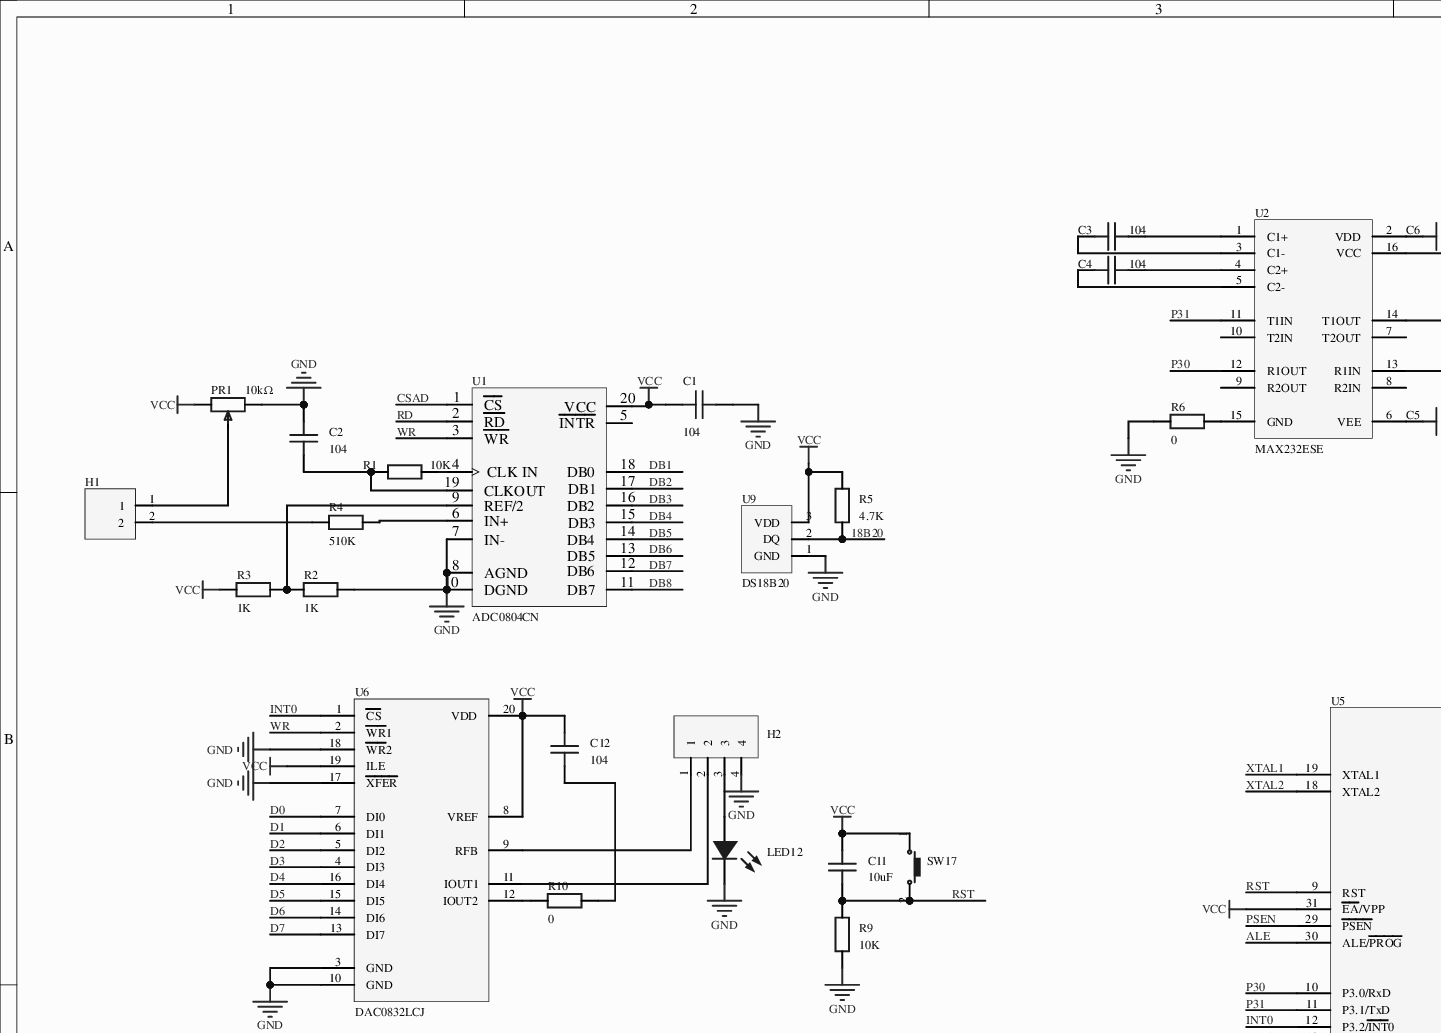
[diagram p0: MISC49866-3.schdoc, top left]
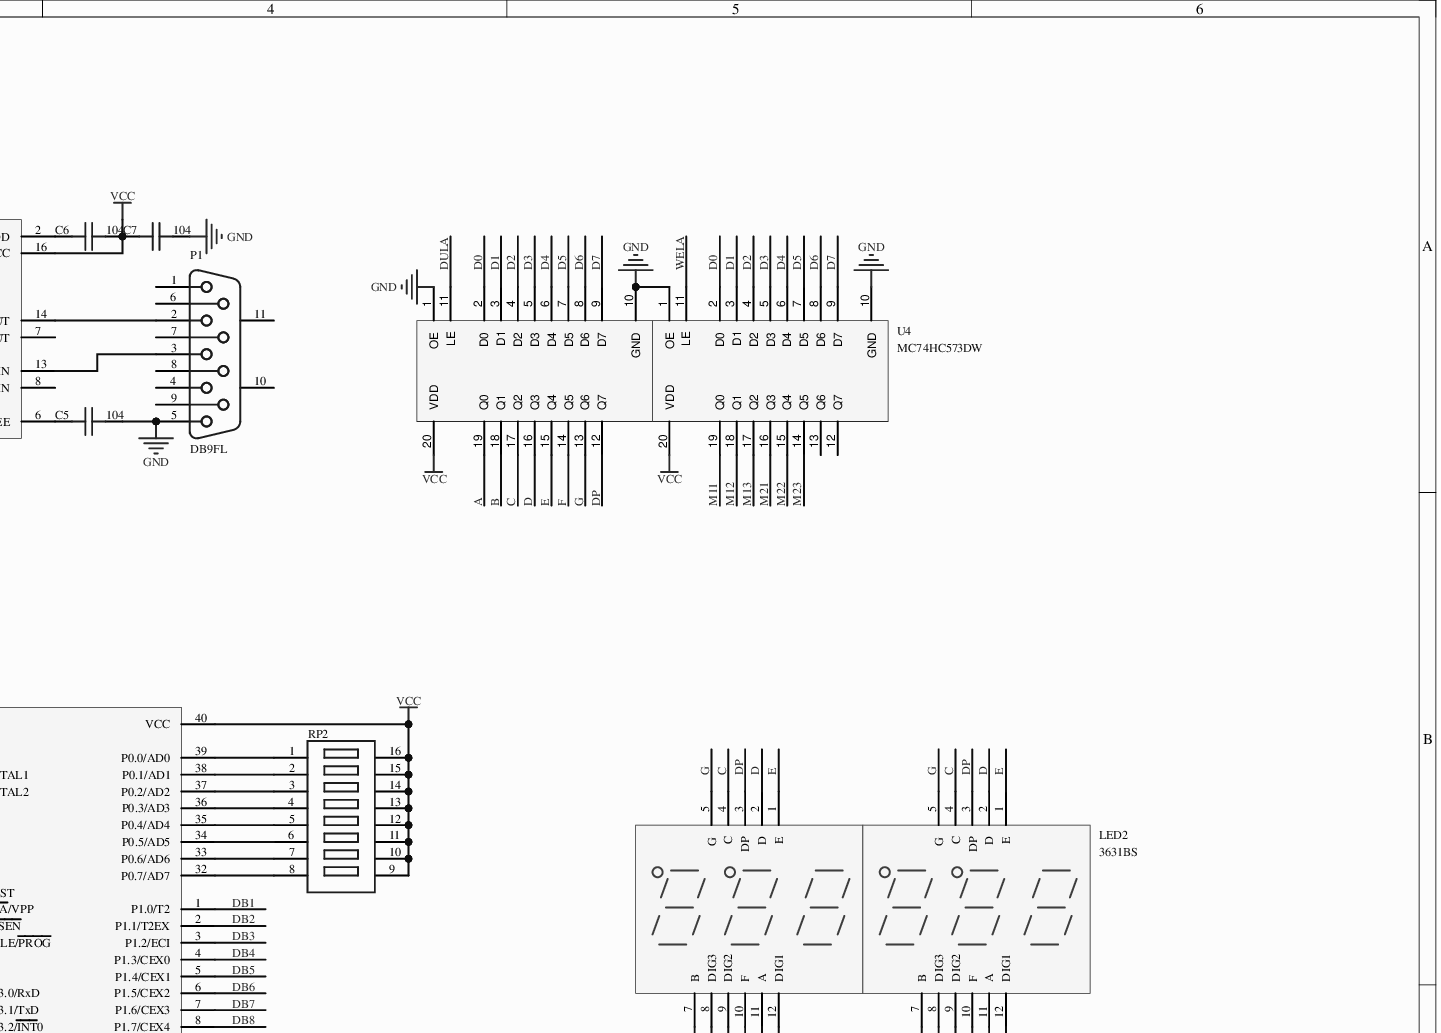
[diagram p1: MISC49866-3.schdoc, top right]
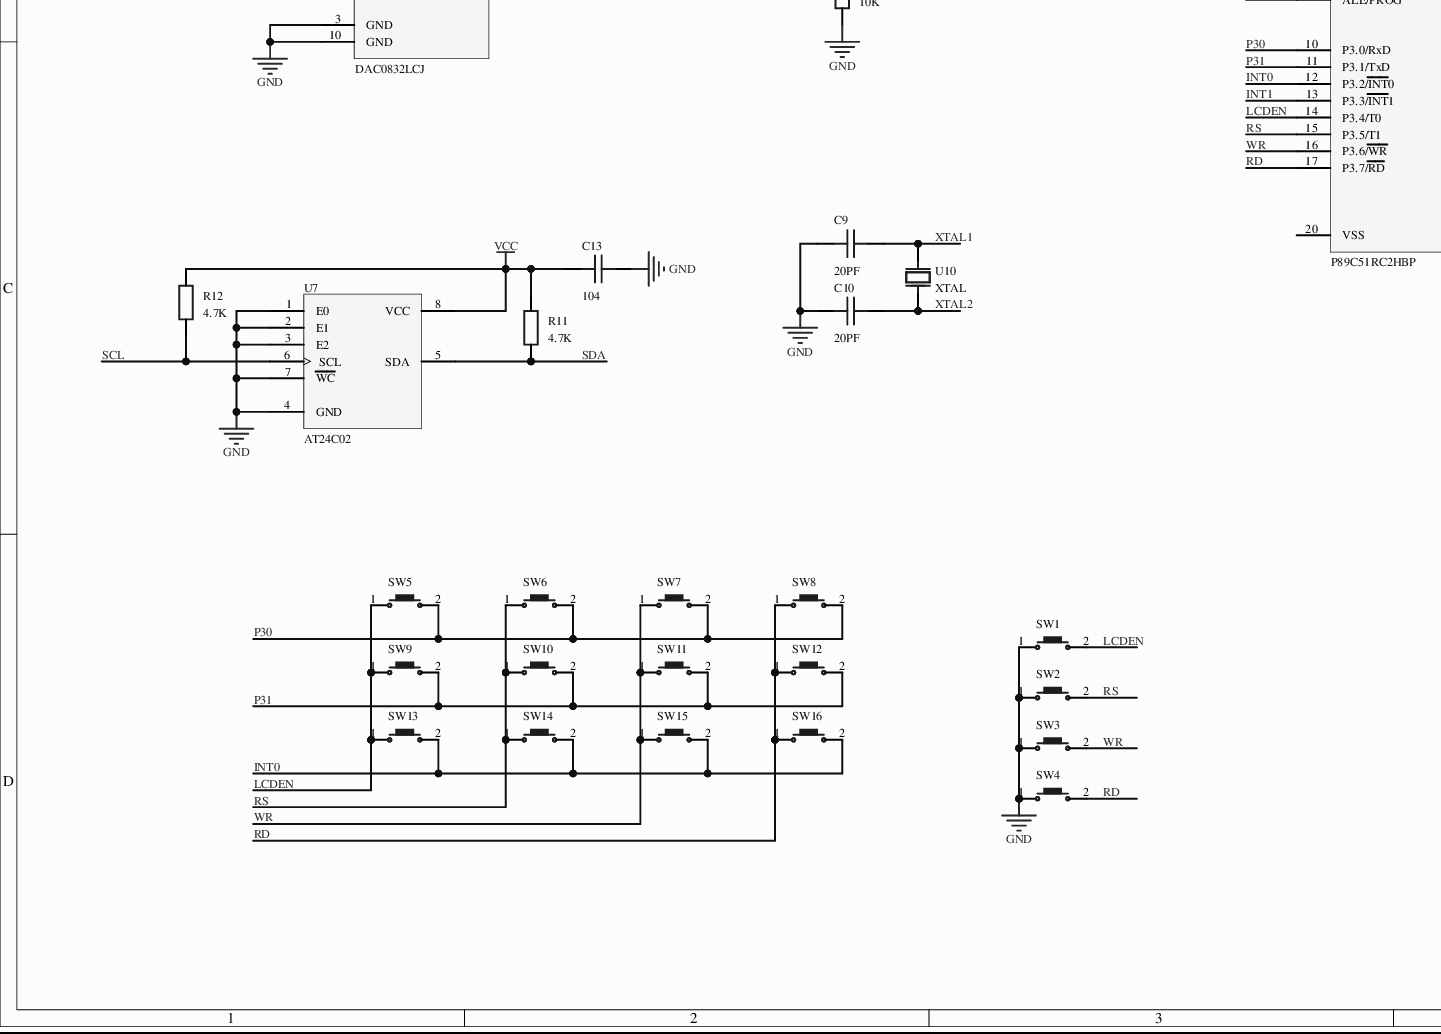
[diagram p2: MISC49866-3.schdoc, bottom left]
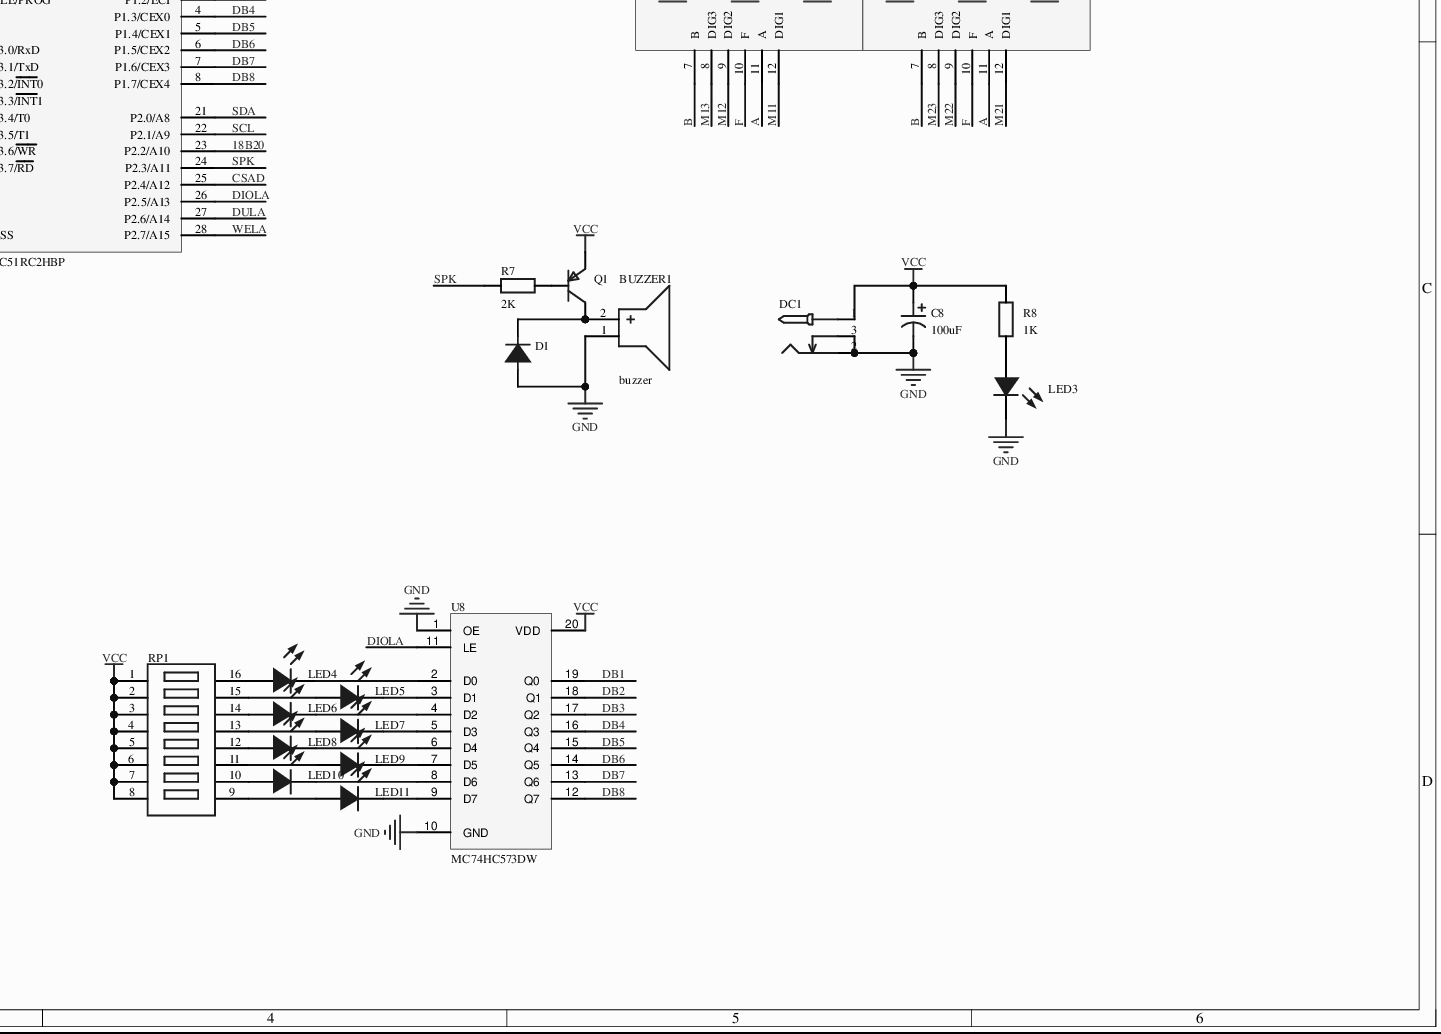
[diagram p3: MISC49866-3.schdoc, bottom right]
# Altium project MISC49866-2.PrjPcb
1 sheet, 74 parts. Net scope: global (net labels, ports and power ports of the same name join across sheets).
Board file: MISC49866.pcbdoc

## Sheet MISC49866-3.schdoc
size 420 x 297 mm; Version: V1.0; @Project Name: MISC49866; @Update Date: 2026-09-29; @Create Date: 2026-09-29; @Board Name: MISC49866; @Create Time: 10:53:11; @Page Count: 1; @Page No: 1; @Schematic Name: MISC49866; @Update Time: 10:53:11; Size: A4

### Parts
BUZZER1  buzzer  [BUZ-TH_BD12.0-P6.00-D0.9-RD]
C1  104  [C0603]
C2  104  [C0603]
C3  104  [C0603]
C4  104  [C0603]
C5  104  [C0603]
C6  104  [C0603]
C7  104  [C0603]
C8  100uF  [CAP-TH_BD5.0-P2.00-D0.8-FD-10UF50VC110GL]
C9  20PF  [C0603]
C10  20PF  [C0603]
C11  10uF  [C0603]
C12  104  [C0603]
C13  104  [C0603]
D1  (no value)  [DO_1N4007]
DC1  (no value)  [DC-005_2.5]
H1  (no value)  [HDR-TH_2P-P2.54-V-M-1]
H2  (no value)  [HDR-TH_4P-P2.54-V-M]
LED1  3631BS  [LED-SEG-TH_11P-L37.5-W19.0-P2.54-LS15.2-BL_1]
LED2  3631BS  [LED-SEG-TH_11P-L37.5-W19.0-P2.54-LS15.2-BL_1]
LED3  (no value)  [LED_0603]
LED4  (no value)  [LED_0603]
LED5  (no value)  [LED_0603]
LED6  (no value)  [LED_0603]
LED7  (no value)  [LED_0603]
LED8  (no value)  [LED_0603]
LED9  (no value)  [LED_0603]
LED10  (no value)  [LED_0603]
LED11  (no value)  [LED_0603]
LED12  (no value)  [LED_0603]
P1  DB9FL  [DB9-TH_DB9F]
PR1  10kΩ  [R_3296]
Q1  (no value)  [S8550P_TO-92]
R1  10K  [R0603]
R2  1K  [R0603]
R3  1K  [R0603]
R4  510K  [R0603]
R5  4.7K  [R0603]
R6  0  [R0603]
R7  2K  [R0603]
R8  1K  [R0603]
R9  10K  [R0603]
R10  0  [R0603]
R11  4.7K  [R0603]
R12  4.7K  [R0603]
RP1  (no value)  [DIP-16_L20.3-W10.2-P2.54-LS7.6-BL]
RP2  (no value)  [DIP-16_L20.3-W10.2-P2.54-LS7.6-BL]
SW1  (no value)  [Key_SMD_3x4x2]
SW2  (no value)  [Key_SMD_3x4x2]
SW3  (no value)  [Key_SMD_3x4x2]
SW4  (no value)  [Key_SMD_3x4x2]
SW5  (no value)  [Key_SMD_3x4x2]
SW6  (no value)  [Key_SMD_3x4x2]
SW7  (no value)  [Key_SMD_3x4x2]
SW8  (no value)  [Key_SMD_3x4x2]
SW9  (no value)  [Key_SMD_3x4x2]
SW10  (no value)  [Key_SMD_3x4x2]
SW11  (no value)  [Key_SMD_3x4x2]
SW12  (no value)  [Key_SMD_3x4x2]
SW13  (no value)  [Key_SMD_3x4x2]
SW14  (no value)  [Key_SMD_3x4x2]
SW15  (no value)  [Key_SMD_3x4x2]
SW16  (no value)  [Key_SMD_3x4x2]
SW17  (no value)  [Key_SMD_3x4x2]
U1  ADC0804CN  [ADC0804CN]
U2  MAX232ESE
U3  MC74HC573DW  (value not drawn)
U4  MC74HC573DW
U5  P89C51RC2HBP
U6  DAC0832LCJ  [J20A]
U7  AT24C02
U8  MC74HC573DW
U9  DS18B20  [TO-92-3_L4.9-W3.7-P1.27-L]
U10  Manufacturer: XTAL  [osc-smd_l3.2-w1.5]  (hidden comment: 32768/10ppm/12.5pF)

### Nets
GND: BUZZER1.1(-) C1.2 C2.2 C5.1 C7.1 C8.2 C9.1 C10.1 C13.2 D1.2(A) DC1.2 DC1.3 H2.4 LED3.1(C) LED12.1(C) P1.5 PR1.3 R2.2 R6.1 R9.1 SW1.1 SW2.1 SW3.1 SW4.1 U1.7(IN-) U1.8(AGND) U1.10(DGND) U3.1(OE) U3.10(GND) U4.1(OE) U4.10(GND) U6.3(GND) U6.10(GND) U6.17(~{XFER}) U6.18(~{WR}2) U7.1(E0) U7.2(E1) U7.3(E2) U7.4(GND) U7.7(~{WC}) U8.1(OE) U8.10(GND) U9.1(GND)
VCC: C1.1 C6.1 C7.2 C8.1 C11.2 C12.2 C13.1 DC1.1 PR1.1 Q1.1(E) R3.1 R5.2 R8.2 R11.2 R12.2 RP1.1 RP1.2 RP1.3 RP1.4 RP1.5 RP1.6 RP1.7 RP1.8 RP2.9 RP2.10 RP2.11 RP2.12 RP2.13 RP2.14 RP2.15 RP2.16 SW17.1 U1.20(VCC) U2.16(VCC) U3.20(VDD) U4.20(VDD) U5.31(~{EA}/VPP) U5.40(VCC) U6.8(VREF) U6.19(ILE) U6.20(VDD) U7.8(VCC) U8.20(VDD) U9.3(VDD)
18B20: R5.1 U5.23(P2.2/A10) U9.2(DQ)
A: LED1.11(A) LED2.11(A) U3.19(Q0)
ALE: U5.30(ALE/~{PROG})
B: LED1.7(B) LED2.7(B) U3.18(Q1)
C: LED1.4(C) LED2.4(C) U3.17(Q2)
CSAD: U1.1(~{CS}) U5.25(P2.4/A12)
D: LED1.2(D) LED2.2(D) U3.16(Q3)
D0: U3.2(D0) U4.2(D0) U6.7(DI0)
D1: U3.3(D1) U4.3(D1) U6.6(DI1)
D2: U3.4(D2) U4.4(D2) U6.5(DI2)
D3: U3.5(D3) U4.5(D3) U6.4(DI3)
D4: U3.6(D4) U4.6(D4) U6.16(DI4)
D5: U3.7(D5) U4.7(D5) U6.15(DI5)
D6: U3.8(D6) U4.8(D6) U6.14(DI6)
D7: U3.9(D7) U4.9(D7) U6.13(DI7)
DB1: U1.18(DB0) U5.1(P1.0/T2) U8.19(Q0)
DB2: U1.17(DB1) U5.2(P1.1/T2EX) U8.18(Q1)
DB3: U1.16(DB2) U5.3(P1.2/ECI) U8.17(Q2)
DB4: U1.15(DB3) U5.4(P1.3/CEX0) U8.16(Q3)
DB5: U1.14(DB4) U5.5(P1.4/CEX1) U8.15(Q4)
DB6: U1.13(DB5) U5.6(P1.5/CEX2) U8.14(Q5)
DB7: U1.12(DB6) U5.7(P1.6/CEX3) U8.13(Q6)
DB8: U1.11(DB7) U5.8(P1.7/CEX4) U8.12(Q7)
DIOLA: U5.26(P2.5/A13) U8.11(LE)
DP: LED1.3(DP) LED2.3(DP) U3.12(Q7)
DULA: U3.11(LE) U5.27(P2.6/A14)
E: LED1.1(E) LED2.1(E) U3.15(Q4)
F: LED1.10(F) LED2.10(F) U3.14(Q5)
G: LED1.5(G) LED2.5(G) U3.13(Q6)
INT0: SW13.2 SW14.2 SW15.2 SW16.2 U5.12(P3.2/~{INT}0) U6.1(~{CS})
INT1: U5.13(P3.3/~{INT}1)
LCDEN: SW1.2 SW5.1 SW9.1 SW13.1 U5.14(P3.4/T0)
M11: LED1.12(DIG1) U4.19(Q0)
M12: LED1.9(DIG2) U4.18(Q1)
M13: LED1.8(DIG3) U4.17(Q2)
M21: LED2.12(DIG1) U4.16(Q3)
M22: LED2.9(DIG2) U4.15(Q4)
M23: LED2.8(DIG3) U4.14(Q5)
P30: SW5.2 SW6.2 SW7.2 SW8.2 U2.12(R1OUT) U5.10(P3.0/RxD)
P31: SW9.2 SW10.2 SW11.2 SW12.2 U2.11(T1IN) U5.11(P3.1/TxD)
PSEN: U5.29(~{PSEN})
RD: SW4.2 SW8.1 SW12.1 SW16.1 U1.2(~{RD}) U5.17(P3.7/~{RD})
RS: SW2.2 SW6.1 SW10.1 SW14.1 U5.15(P3.5/T1)
RST: C11.1 R9.2 SW17.2 U5.9(RST)
SCL: R12.1 U5.22(P2.1/A9) U7.6(SCL)
SDA: R11.1 U5.21(P2.0/A8) U7.5(SDA)
SPK: R7.1 U5.24(P2.3/A11)
WELA: U4.11(LE) U5.28(P2.7/A15)
WR: SW3.2 SW7.1 SW11.1 SW15.1 U1.3(~{WR}) U5.16(P3.6/~{WR}) U6.2(~{WR}1)
XTAL1: C9.2 U5.19(XTAL1) U10.2(OSC2)
XTAL2: C10.2 U5.18(XTAL2) U10.1(OSC1)
NetBUZZER1_2: BUZZER1.2(+) D1.1(K) Q1.3(C)
NetC2_1: C2.1 R1.1 U1.19(CLKOUT)
NetC3_1: C3.1 U2.1(C1+)
NetC3_2: C3.2 U2.3(C1-)
NetC4_1: C4.1 U2.4(C2+)
NetC4_2: C4.2 U2.5(C2-)
NetC5_2: C5.2 U2.6(VEE)
NetC6_2: C6.2 U2.2(VDD)
NetC12_1: C12.1 R10.2
NetH1_1: H1.1 PR1.2
NetH1_2: H1.2 R4.1
NetH2_1: H2.1 U6.9(RFB)
NetH2_2: H2.2 U6.11(IOUT1)
NetH2_3: H2.3 LED12.2(A)
NetLED3_2: LED3.2(A) R8.1
NetLED4_1: LED4.1(C) U8.2(D0)
NetLED4_2: LED4.2(A) RP1.16
NetLED5_1: LED5.1(C) U8.3(D1)
NetLED5_2: LED5.2(A) RP1.15
NetLED6_1: LED6.1(C) U8.4(D2)
NetLED6_2: LED6.2(A) RP1.14
NetLED7_1: LED7.1(C) U8.5(D3)
NetLED7_2: LED7.2(A) RP1.13
NetLED8_1: LED8.1(C) U8.6(D4)
NetLED8_2: LED8.2(A) RP1.12
NetLED9_1: LED9.1(C) U8.7(D5)
NetLED9_2: LED9.2(A) RP1.11
NetLED10_1: LED10.1(C) U8.8(D6)
NetLED10_2: LED10.2(A) RP1.10
NetLED11_1: LED11.1(C) U8.9(D7)
NetLED11_2: LED11.2(A) RP1.9
NetP1_2: P1.2 U2.14(T1OUT)
NetP1_3: P1.3 U2.13(R1IN)
NetQ1_2: Q1.2(B) R7.2
NetR1_2: R1.2 U1.4(CLK_IN)
NetR2_1: R2.1 R3.2 U1.9(REF/2)
NetR4_2: R4.2 U1.6(IN+)
NetR6_2: R6.2 U2.15(GND)
NetR10_1: R10.1 U6.12(IOUT2)
NetRP2_1: RP2.1 U5.39(P0.0/AD0)
NetRP2_2: RP2.2 U5.38(P0.1/AD1)
NetRP2_3: RP2.3 U5.37(P0.2/AD2)
NetRP2_4: RP2.4 U5.36(P0.3/AD3)
NetRP2_5: RP2.5 U5.35(P0.4/AD4)
NetRP2_6: RP2.6 U5.34(P0.5/AD5)
NetRP2_7: RP2.7 U5.33(P0.6/AD6)
NetRP2_8: RP2.8 U5.32(P0.7/AD7)

Not connected (* = marked no-connect by the designer): P1 1* 4* 6* 7* 8* 9* 10(MH1)* 11(MH2)*; U1 5(~{INTR})*; U2 7(T2OUT)* 8(R2IN)* 9(R2OUT)* 10(T2IN)*; U4 12(Q7)* 13(Q6)*; U5 20(VSS)*

### Library data of the parts
BUZZER1 = buzzer: AddInBom: yes; ModelId: af17e4151ed84fc2a628230bf23763630819f05c4eef4c71ace90d822a990e87; ModelTransform: 472.44,472.176,0,270,0,0,0,0,-196.85; Symbol: BUZZER; Device: buzzer; FootprintName: BUZ-TH_BD12.0-P6.00-D0.9-RD; LCSC Part Name: buzzer; SupplierPart: C9900014030; ManufacturerPart: buzzer; Supplier Footprint: buzzer; JLCPCB Part Class: Extended Part; Supplier: LCSC; ConvertToPcb: yes; ModelName: BUZ-TH_BD12.0-P6.00-D0.9-RD
C1-C7 C9-C13 = CAP_0603: Symbol: Capacitance; ConvertToPcb: yes; ModelId: ac125912035d415993ca9572d50418b10819f05c4eef4c71ace90d822a990e87; ModelName: C0603_L1.6-W0.8-H0.8; ModelTransform: 62.992,31.496,0,0,0,0,0,0,0; Device: CAP_0603; FootprintName: C0603; AddInBom: yes; Supplier Footprint: 0603
  C1-C7 C12 C13: Value: 104
  C9 C10: Value: 20PF
  C11: Value: 10uF
C8 = 10UF50VC110GL: Capacitance: 10uF; tolerance: ±20%; rated voltage: 50V; ripple current: 120mA@100KHz; equivalent series resistance (ESR): 1.6Ω;; Manufacturer: Econd(米朗电子); AddInBom: yes; ModelId: b35ab6b0460c4c43a629d91cfc2b58780819f05c4eef4c71ace90d822a990e87; ModelTransform: 196.85,196.85,0,0,0,0,0,0,-196.85; Pin Spacing: 2mm; Lifetime: 5000hrs@105℃; Symbol: 10UF50VC110GL; Device: 10UF50VC110GL; Value: 100uF; FootprintName: CAP-TH_BD5.0-P2.00-D0.8-FD-10UF50VC110GL; LCSC Part Name: 10uF ±20% 50V; ManufacturerPart: 10UF50VC110GL; Supplier Footprint: 插件,D5xL11mm; JLCPCB Part Class: Extended Part; Datasheet: https://item.szlcsc.com/datasheet/10UF50VC110GL/49031974.html; Supplier: LCSC; ConvertToPcb: yes; ModelName: CAP-TH_BD5.0-P2.00-D0.8-FD-10UF50VC110GL; Tolerance: ±20%; Voltage Rating: 50V; Ripple Current: 120mA@100KHz; Equivalent Series Resistance(ESR): 1.6Ω; Diameter: 5mm; Height - Seated (Max): 11mm; Operating Temperature: -40℃~+105℃
D1 = D_1N4007A: AddInBom: yes; ModelId: 6de1e9b71a0d4751b4e9df530304c1a30819f05c4eef4c71ace90d822a990e87; ModelName: DO-41_D2.4-L4.7-P8.70; ModelTransform: 373.9,94.4,232.29,0,0,0,0,0,-140; Symbol: D_1N4007; Device: D_1N4007A; FootprintName: DO_1N4007; Supplier Footprint: DO-41; ConvertToPcb: yes
DC1 = DC-005_2.5: ConvertToPcb: yes; ModelId: f168fe383f964e0ea2af0127ff6ac7b40819f05c4eef4c71ace90d822a990e87; ModelName: DC-IN-TH_DC005; ModelTransform: 366.14,553.15,590.55,90,0,0,137.8,-11.81,-157.48; Symbol: DC-005_2.5; Device: DC-005_2.5; FootprintName: DC-005_2.5; AddInBom: yes; Supplier Footprint: 插件
H1 = HDR-M_2.54_1x2P: Symbol: 210S-1*2P L=11.6MMGold-plated black; ConvertToPcb: yes; ModelId: 79b2e9f2d70a4d68a1b7098f27c6d4c50819f05c4eef4c71ace90d822a990e87; ModelName: HDR-M-2.54_1x2; ModelTransform: 200,100,0,0,0,0,0,0,-118.11; Device: HDR-M_2.54_1x2P; FootprintName: HDR-TH_2P-P2.54-V-M-1; AddInBom: yes; SupplierPart: C124375; Supplier Footprint: 插件
H2 = HDR-M_2.54_1x4P: Symbol: PZ254V-11-04P; ConvertToPcb: yes; ModelId: 112f4d05e8d64e99ab9a333894bea4f90819f05c4eef4c71ace90d822a990e87; ModelName: HDR-TH_4P-P2.54-M-LI-1X4P; ModelTransform: 399.999,104.7242,0,0,0,0,0,0,-118.11; Device: HDR-M_2.54_1x4P; FootprintName: HDR-TH_4P-P2.54-V-M; AddInBom: yes; SupplierPart: C492403; Supplier Footprint: 插件
LED1 LED2 = 3631BS: Digit count: 3; luminous colour: blue; LED polarity: common anode; digit/letter size (inch): 0.56;; Manufacturer: 志浩; Number of Characters: 3 digits; Digit/Alpha Size(inch): 0.56; 3D Model: f54e6f5f8ebd42c59fa542745733582317bf92a994fa409e84525e65b42a2577; 3D Model Transform: 1476.375,748.424,0,0,0,0,0,0,-157.48; AddInBom: yes; Symbol: 3631BS; Device: 3631BS; LCSC Part Name: 3位0.56英寸 蓝光共阳 数码管; Supplier Part: C2938341; Manufacturer Part: 3631BS; Supplier Footprint: 插件; JLCPCB Part Class: Extended library; Datasheet: https://atta.szlcsc.com/upload/public/pdf/source/20220104/5C2FBAA78B63B49D128F0D9B62C0A18B.pdf; Supplier: LCSC; Luminous Color: Blue; LED Polarity: Common anode; FootprintName: LED-SEG-TH_11P-L37.5-W19.0-P2.54-LS15.2-BL_1; ConvertToPcb: yes; ModelName: LED-SEG-TH_11P-L37.5-W19.0-P2.54-LS15.2-BL_1
LED3-LED12 = LED_0603-B: Symbol: LED_B; Convert to PCB: yes; 3D Model: eb8d964598f24248affda46f619856c50819f05c4eef4c71ace90d822a990e87; 3D Model Transform: 63.1,31.6,23.7,0,0,0,0,0,0; ModelName: LED-0603_B; Device: LED_0603-B; Add into BOM: yes; Supplier Footprint: 0603; FootprintName: LED_0603
P1 = DB9FL: AddInBom: yes; ModelId: fd27160e2e724a89a2372c6f814078df314da64f82a2492c9607ff1f6bb3435e; ModelName: DB9-TH_DB9-H-F_C2888345; ModelTransform: 1212.596,700.786,0,0,0,0,0,-230.315,-177.165; Symbol: DB9FL; Device: DB9FL; FootprintName: DB9-TH_DB9F; LCSC Part Name: DB9FL; SupplierPart: C9900001807; ManufacturerPart: DB9FL; Supplier Footprint: DConnector9; JLCPCB Part Class: Extended library; Supplier: LCSC; ConvertToPcb: yes
PR1 = R_3296: ConvertToPcb: yes; ModelId: b182808559bb43bda9e7de64b64134cb0819f05c4eef4c71ace90d822a990e87; ModelName: 3296W; ModelTransform: 373.98,188.96,590.49,180,0,0,0,0,-140; Symbol: R_3296; Device: R_3296; FootprintName: R_3296; AddInBom: yes; Supplier Footprint: 直插; Value: 10kΩ
Q1 = S8550_TO_PNP: ConvertToPcb: yes; ModelId: aafe8e06f2154e7c93506efd0d6632dd0819f05c4eef4c71ace90d822a990e87; ModelName: TO-92-3_L4.9-W3.7-P1.27-L; ModelTransform: 180.78,141.44,417.3,0,0,0,0,0,-200; Symbol: S8550_TO_PNP; Device: S8550_TO_PNP; FootprintName: S8550P_TO-92; AddInBom: yes; Supplier Footprint: TO-92
R1-R12 = Res_0603: Symbol: Resistor; ConvertToPcb: yes; ModelId: fc143cca1e79419f9cd78b61e9279f080819f05c4eef4c71ace90d822a990e87; ModelTransform: 31.8897,63.7794,0,90,0,0,0,0,0; Device: Res_0603; FootprintName: R0603; AddInBom: yes; Supplier Footprint: 0603; ModelName: R0603
  R1 R9: Value: 10K
  R2 R3 R8: Value: 1K
  R4: Value: 510K
  R5 R11 R12: Value: 4.7K
  R6 R10: Value: 0
  R7: Value: 2K
RP1 RP2 = paizu: AddInBom: yes; ModelId: b73b726218474b419f7d257eb9cc4370d07147df35bb4ee1ae33039552c243e2; ModelName: DIP-16_L20.3-W10.2-P2.54-LS7.6-BL-1; ModelTransform: 799.998,399.999,0,0,0,0,0,0,-118.11; Symbol: paizu; Device: paizu; ConvertToPcb: yes; FootprintName: DIP-16_L20.3-W10.2-P2.54-LS7.6-BL
SW1-SW17 = Key_SMD_3x4x2: Symbol: Tact switch x2; ConvertToPcb: yes; ModelId: 63599cce708d48afbce1b0db003544770819f05c4eef4c71ace90d822a990e87; ModelName: SW-SMD_L4.0-W2.9-H2-LS5.0; ModelTransform: 196.85,114.17,79.13,0,0,0,0,0,0; Device: Key_SMD_3x4x2; FootprintName: Key_SMD_3x4x2; AddInBom: yes; Supplier Footprint: SMD
U1 = ADC0804CN: AddInBom: yes; Symbol: ADC0804CN; Device: ADC0804CN; FootprintName: ADC0804CN; ConvertToPcb: yes
U2 = MAX232ESE: RS232; Package1: SOIC-16_150mil; AddInBom: yes; Symbol: MAX232ESE; Device: MAX232ESE; ComponentLink1Description: Supplier link; Supplier: LC; SuppliersPartNumber: C26860; Footprint Name: LC-SOIC-16_150mil; ConvertToPcb: yes
U3 U4 U8 = MC74HC573DW: ConvertToPcb: yes; Symbol: MC74HC573DW; Device: MC74HC573DW; AddInBom: yes
U5 = P89C51RC2HBP: AddInBom: yes; Symbol: P89C51RC2HBP; Device: P89C51RC2HBP; ConvertToPcb: yes
U6 = DAC0832LCJ: ComponentAvailability: Obsolete; AddInBom: yes; Symbol: DAC0832LCJ; Device: DAC0832LCJ; Published: 15-Apr-2002; LatestRevisionDate: 06-Jun-2005; LatestRevisionNote: Stylized 3D Model Added.; DatasheetVersion: May-1999; PackageVersion: 2000; PackageReference: J20A; PackageDescription: DIP; 20 Leads; Row Spacing 7.62 mm; Pitch 2.54 mm; Code_JEDEC: MS-015-AE; ComponentLink1Description: Manufacturer Link; ComponentLink2Description: Datasheet; ComponentLink3Description: Discontinuation Notice; ComponentLink4Description: URL Link1; ConvertToPcb: yes; FootprintName: J20A; Publisher: Altium Limited
U7 = M24C02BN6: AddInBom: yes; Origin Footprint 2: PSDIP8A; Origin Footprint 3: SOP8_L; Origin Footprint 4: SOP8_N; Origin Footprint 5: AT24CB; Origin Footprint 6: DIP8; Symbol: M24C02BN6; Device: M24C02BN6; ConvertToPcb: yes; Published: 24-Aug-2001; LatestRevisionDate: 06-Jun-2005; LatestRevisionNote: Stylized 3D Model Added.; DatasheetVersion: Sep-1999; PackageVersion: Jun-1998; PackageReference: PSDIP8A; PackageDescription: DIP; 8 Leads; Row Spacing 7.62 mm; Pitch 2.54 mm; ComponentLink1Description: Manufacturer Link; ComponentLink2Description: Datasheet; ComponentLink2URL: http://www.st.com/stonline/products/literature/ds/5067/m24c01-r.pdf; Publisher: Altium Limited
U9 = DS18B20: Manufacturer: Youtai Semiconductor Co., Ltd.; AddInBom: yes; ModelId: aafe8e06f2154e7c93506efd0d6632ddc675cafc06334f02bb6e99fe0a86729f; Symbol: DS18B20; Device: DS18B20; FootprintName: TO-92-3_L4.9-W3.7-P1.27-L; Supplier: LCSC; SupplierPart: C376006; ManufacturerPart: DS18B20; JLCPCB Part Class: Extended Part; ConvertToPcb: yes; ModelName: TO-92-3_L4.9-W3.7-P1.27-L
U10 = 32768/10ppm/12.5pF: AddInBom: yes; ModelId: 2dd241c0893b4675b8def6f6998a8251343fa624c39949f9abdc5569de48b688; ModelName: OSC-SMD_L3.2-W1.5-H0.8; ModelTransform: 125.984,59.055,0,0,0,0,0,0,0; Symbol: 32768/10ppm/12.5pf; Device: 32768/10ppm/12.5pF; FootprintName: osc-smd_l3.2-w1.5; LCSC Part Name: 32768/10ppm/12.5pF; SupplierPart: C9900093280; ManufacturerPart: 32768/10ppm/12.5pF; Supplier Footprint: XTAL3215; JLCPCB Part Class: Extended library; Supplier: LCSC; ConvertToPcb: yes